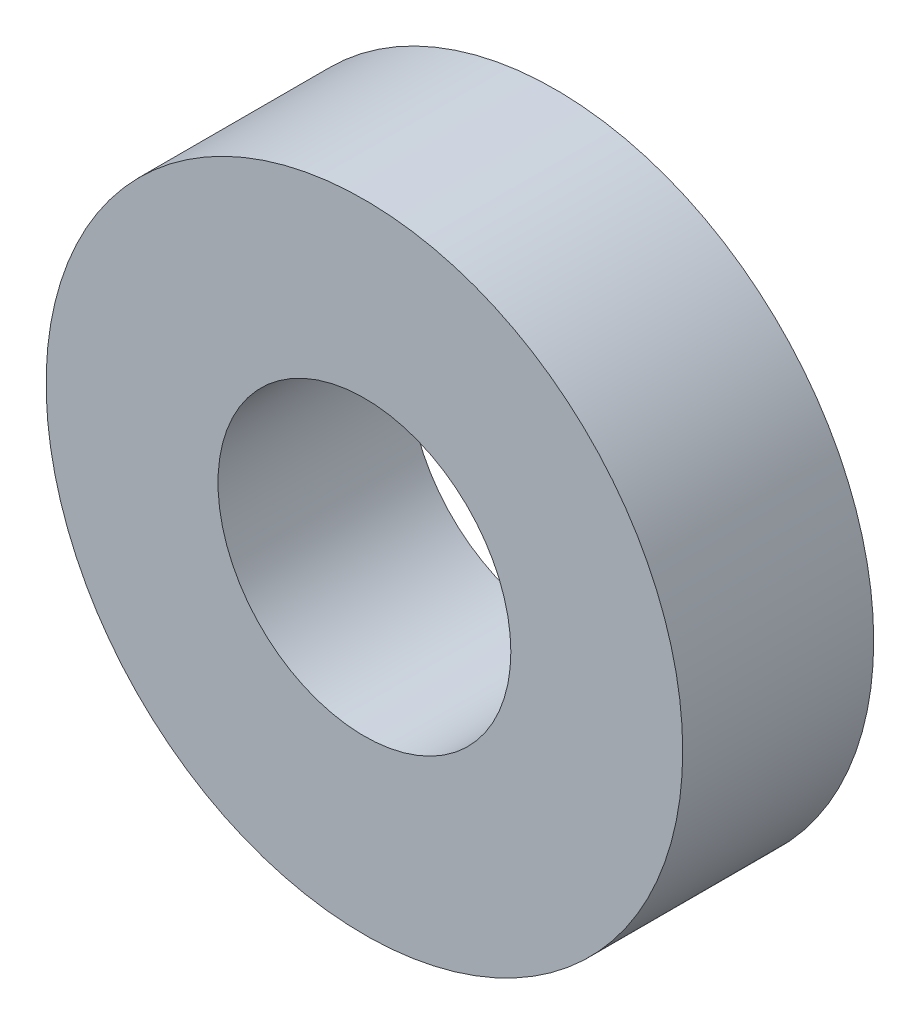
SolidWorks part; units mm, degrees
ref_plane "Front Plane" through (0, 0, 0) normal (0, 0, 1) x (1, 0, 0)
ref_plane "Top Plane" through (0, 0, 0) normal (0, 1, 0) x (1, 0, 0)
ref_plane "Right Plane" through (0, 0, 0) normal (1, 0, 0) x (0, 0, -1)
sketch "Sketch1" plane through (0, 0, 0) normal (0, 0, 1) x (1, 0, 0)
  circle A0 centre (0, 0) radius 2.3
  circle A1 centre (0, 0) radius 5
  dimension "D1" = 4.6
  dimension "D2" = 10
extrude "Boss-Extrude1" add sketch "Sketch1" along normal blind 3
